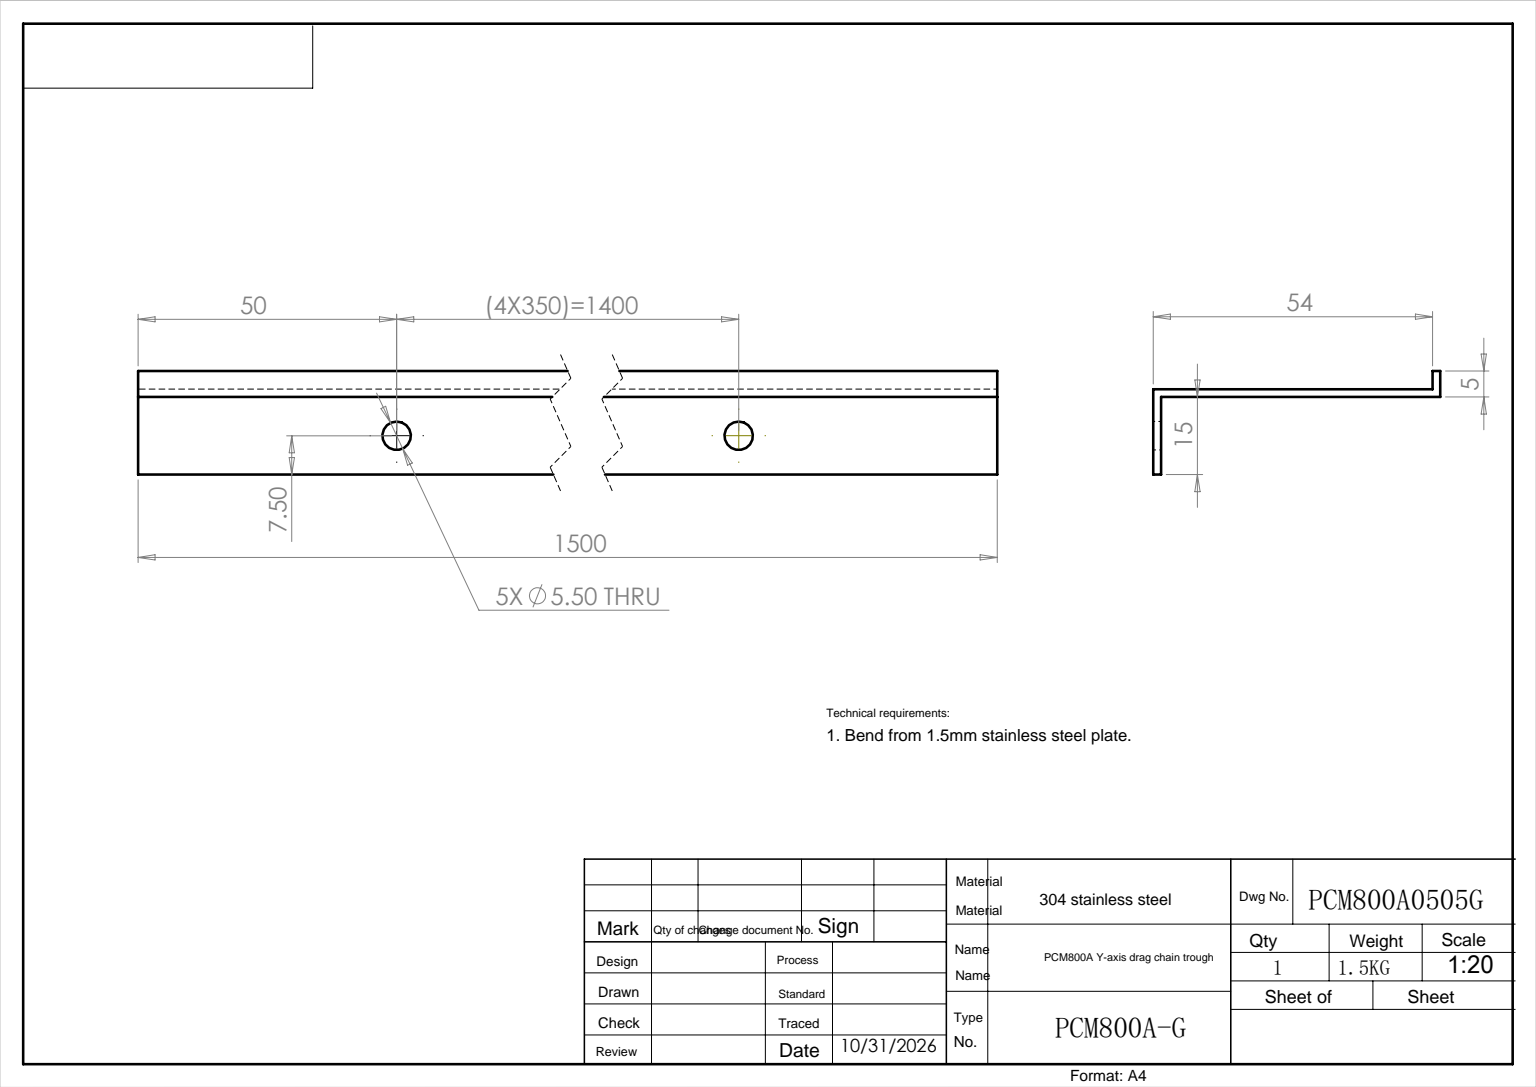
SolidWorks part; units mm, degrees
ref_plane "前视基准面" through (0, 0, 0) normal (0, 0, 1) x (1, 0, 0)
ref_plane "上视基准面" through (0, 0, 0) normal (0, 1, 0) x (1, 0, 0)
ref_plane "右视基准面" through (0, 0, 0) normal (1, 0, 0) x (0, 0, -1)
sketch "草图1" plane through (0, 0, 0) normal (0, 0, 1) x (1, 0, 0)
  line L0 (0, 0) -> (0, -15)
  line L1 (0, 0) -> (54, 0)
  line L2 (54, 0) -> (54, 5)
  dimension "D1" = 5
  dimension "D2" = 15
  dimension "D3" = 54
extrude "拉伸-薄壁1" add sketch "草图1" along normal blind 1500 thin
sketch "草图2" plane through (0, 0, 0) normal (1, 0, 0) x (0, 0, -1)
  line L0 (-1500, -7.5) -> (113.6308, -7.5) construction
  line L1 (-1500, -15) -> (-1500, 0) construction
  circle A0 centre (-1450, -7.5) radius 2.75
  circle A1 centre (-1100, -7.5) radius 2.75
  circle A2 centre (-750, -7.5) radius 2.75
  circle A3 centre (-400, -7.5) radius 2.75
  circle A4 centre (-50, -7.5) radius 2.75
  dimension "D1" = 5.5
  dimension "D2" = 50
  dimension "D3" = 5
extrude "切除-拉伸1" cut sketch "草图2" against normal blind 10
